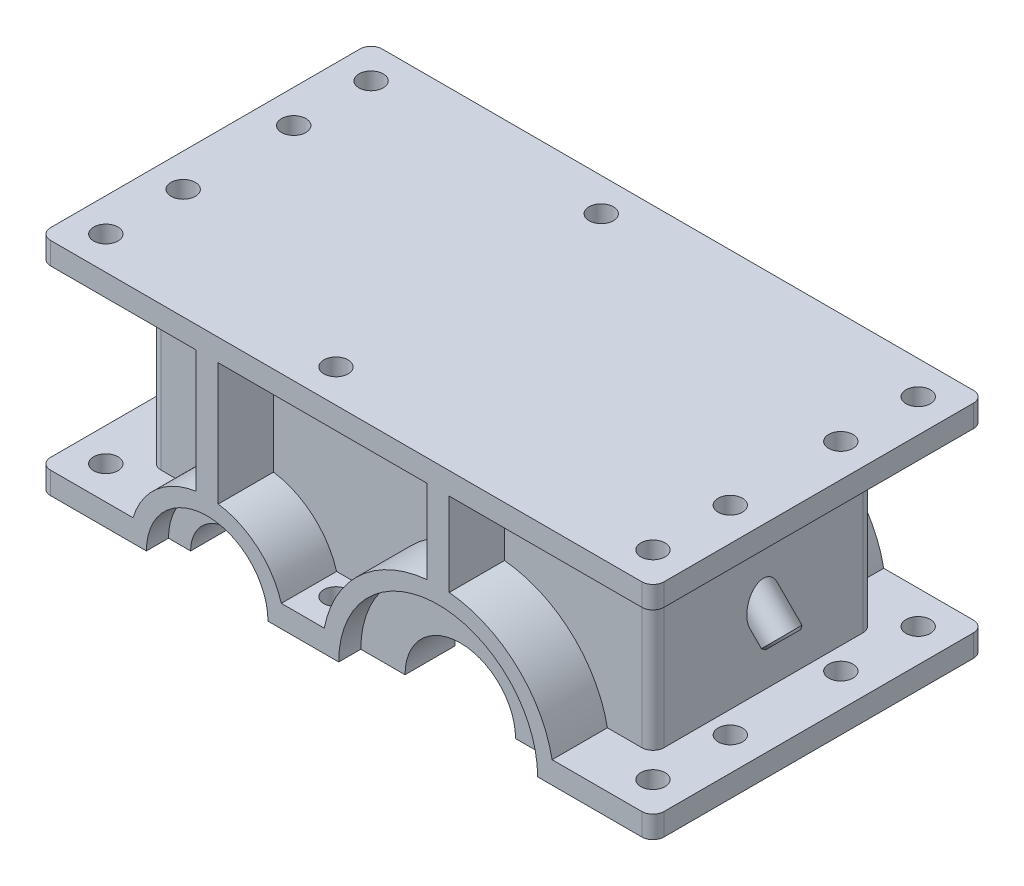
SolidWorks part; units mm, degrees
ref_plane "Front Plane" through (0, 0, 0) normal (0, 0, 1) x (1, 0, 0)
ref_plane "Top Plane" through (0, 0, 0) normal (0, 1, 0) x (1, 0, 0)
ref_plane "Right Plane" through (0, 0, 0) normal (1, 0, 0) x (0, 0, -1)
sketch "Sketch1" plane through (0, 0, 0) normal (0, 0, 1) x (1, 0, 0)
  line L0 (-200, 0) -> (255, 0) construction
  line L1 (0, 200) -> (0, -201.1908) construction
  line L2 (-200, 200) -> (-200, 0)
  line L3 (255, 0) -> (255, 200)
  line L4 (-14.196, 0) -> (-14.196, 143.4811) construction
  line L5 (-200, 0) -> (255, 0)
  line L6 (255, 200) -> (-200, 200)
  circle A0 centre (-98.2783, 0) radius 84 construction
  circle A1 centre (110.7228, 0) radius 125 construction
  dimension "D1" = 250
  dimension "D2" = 110.7228
  dimension "D3" = 168
  dimension "D4" = 209.0011
  dimension "D5" = 200
  dimension "D7" = 200
  dimension "D8" = 255
extrude "Boss-Extrude1" add sketch "Sketch1" along normal mid plane 200
shell "Shell1" thickness 15
sketch "Sketch2" plane through (0, 0, 0) normal (0, 1, 0) x (1, 0, 0)
  line L8 (-114.9858, 100) -> (-200, 100)
  line L9 (54.3355, 100) -> (-114.9858, 100)
  line L10 (255, 100) -> (54.3355, 100)
  line L11 (255, -100) -> (255, 100)
  line L12 (54.3355, -100) -> (255, -100)
  line L13 (-114.9858, -100) -> (54.3355, -100)
  line L14 (-200, -100) -> (-114.9858, -100)
  line L15 (-200, -100) -> (-200, 100)
  line L16 (-114.9858, 150) -> (-250, 150)
  line L17 (-250, -150) -> (-250, 150)
  line L18 (-250, -150) -> (-114.9858, -150)
  line L19 (-114.9858, -150) -> (54.3355, -150)
  line L20 (54.3355, -150) -> (305, -150)
  line L21 (305, -150) -> (305, 150)
  line L22 (305, 150) -> (54.3355, 150)
  line L23 (54.3355, 150) -> (-114.9858, 150)
  dimension "D1" = 50
extrude "Boss-Extrude2" add sketch "Sketch2" along normal blind 20
sketch "Sketch3" plane through (0, 0, 100) normal (0, 0, 1) x (1, 0, 0)
  line L0 (-168.2783, 0) -> (-28.2783, 0)
  line L1 (5.7228, 0) -> (215.7228, 0)
  arc A0 (-28.2783, 0) -> (-168.2783, 0) centre (-98.2783, 0) ccw
  arc A1 (215.7228, 0) -> (5.7228, 0) centre (110.7228, 0) ccw
  line M2 (-200, 20) -> (255, 20)
  dimension "D1" = 105
  dimension "D2" = 70
extrude "Boss-Extrude3" add sketch "Sketch3" along normal blind 50 contours A1 M2 | A0 M2
sketch "Sketch4" plane through (0, 0, 150) normal (0, 0, 1) x (1, 0, 0)
  line L0 (-98.2783, 55) -> (-98.2783, 70) construction
  line L1 (110.7228, 90) -> (110.7228, 105) construction
  circle A0 centre (110.7228, 0) radius 90
  circle A1 centre (-98.2783, 0) radius 55
  arc A2 (-31.1963, 20) -> (-165.3604, 20) centre (-98.2783, 0) ccw construction
  arc A3 (213.8004, 20) -> (7.6451, 20) centre (110.7228, 0) ccw construction
  dimension "D1" = 110
  dimension "D2" = 180
extrude "Cut-Extrude1" cut sketch "Sketch4" against normal blind 20
mirror "Mirror1" about plane through (0, 0, 0) normal (0, 0, 1) of "Cut-Extrude1", "Boss-Extrude3"
sketch "Sketch5" plane through (0, 0, 130) normal (0, 0, 1) x (1, 0, 0)
  circle A0 centre (-98.2783, 0) radius 35
  circle A1 centre (110.7228, 0) radius 50
  dimension "D1" = 70
  dimension "D2" = 100
extrude "Cut-Extrude3" cut sketch "Sketch5" against normal through all
fillet "Fillet1" radius 10 8 edges at (305, 10, 150) (305, 10, -150) (-250, 10, -150) (-250, 10, 150) (-200, 110, -100) (255, 110, -100) (255, 110, 100) (-200, 110, 100)
sketch "Sketch6" plane through (0, 20, 0) normal (0, 1, 0) x (1, 0, 0)
  line L0 (-250, 0) -> (305, 0) construction
  line L1 (-220, 120) -> (-220, 150) construction
  line L2 (-165.3604, 150) -> (-240, 150) construction
  line L3 (-220, 120) -> (-250, 120) construction
  line L4 (-250, 140) -> (-250, -140) construction
  line L5 (-220, -120) -> (-250, -120) construction
  line L6 (-220, -120) -> (-220, -150) construction
  line L7 (305, -140) -> (305, 140) construction
  line L8 (27.5, 0) -> (27.5, 385.3878) construction
  line L9 (275, -120) -> (275, -150) construction
  line L10 (275, -120) -> (305, -120) construction
  line L11 (275, 120) -> (305, 120) construction
  line L12 (275, 120) -> (275, 150) construction
  line L13 (-11.7756, 100) -> (-11.7756, 150) construction
  line L14 (7.6451, 100) -> (-31.1963, 100) construction
  line L15 (7.6451, 150) -> (-31.1963, 150) construction
  line L16 (-250, 120) -> (305, 120) construction
  circle A0 centre (-220, 120) radius 11
  circle A1 centre (-220, 50) radius 11
  circle A2 centre (-220, -50) radius 11
  circle A3 centre (-220, -120) radius 11
  circle A4 centre (275, -120) radius 11
  circle A5 centre (275, -50) radius 11
  circle A6 centre (275, 50) radius 11
  circle A7 centre (275, 120) radius 11
  circle A8 centre (-11.7756, 120) radius 11
  circle A9 centre (-11.7756, -120) radius 11
  dimension "D1" = 22
  dimension "D4" = 22
  dimension "D6" = 22
  dimension "D2" = 30
  dimension "D3" = 30
  dimension "D5" = 70
extrude "Cut-Extrude4" cut sketch "Sketch6" against normal blind 30
sketch "Sketch7" plane through (0, 200, 0) normal (0, 1, 0) x (1, 0, 0)
  line L0 (-165.3604, 150) -> (-240, 150) construction
  line L1 (-250, 140) -> (-250, -140) construction
  line L2 (-240, -150) -> (-165.3604, -150) construction
  line L3 (-165.3604, -150) -> (-31.1963, -150) construction
  line L4 (245, 100) -> (-190, 100)
  line L5 (-200, 90) -> (-200, -90)
  line L6 (-190, -100) -> (245, -100)
  line L7 (255, -90) -> (255, 90)
  line L8 (245, 100) -> (-190, 100)
  line L9 (-200, 90) -> (-200, -90)
  line L10 (-190, -100) -> (245, -100)
  line L11 (255, -90) -> (255, 90)
  line L12 (-31.1963, -150) -> (7.6451, -150) construction
  line L13 (7.6451, -150) -> (213.8004, -150) construction
  line L14 (213.8004, -150) -> (295, -150) construction
  line L15 (305, -140) -> (305, 140) construction
  line L16 (295, 150) -> (213.8004, 150) construction
  line L17 (213.8004, 150) -> (7.6451, 150) construction
  line L18 (7.6451, 150) -> (-31.1963, 150) construction
  line L19 (-31.1963, 150) -> (-165.3604, 150) construction
  line L20 (-165.3604, 150) -> (-240, 150)
  line L21 (-250, 140) -> (-250, -140)
  line L22 (-240, -150) -> (-165.3604, -150)
  line L23 (-165.3604, -150) -> (-31.1963, -150)
  line L24 (-31.1963, -150) -> (7.6451, -150)
  line L25 (7.6451, -150) -> (213.8004, -150)
  line L26 (213.8004, -150) -> (295, -150)
  line L27 (305, -140) -> (305, 140)
  line L28 (295, 150) -> (213.8004, 150)
  line L29 (213.8004, 150) -> (7.6451, 150)
  line L30 (7.6451, 150) -> (-31.1963, 150)
  line L31 (-31.1963, 150) -> (-165.3604, 150)
  arc A0 (-240, 150) -> (-250, 140) centre (-240, 140) ccw construction
  arc A1 (-250, -140) -> (-240, -150) centre (-240, -140) ccw construction
  arc A2 (295, -150) -> (305, -140) centre (295, -140) ccw construction
  arc A3 (305, 140) -> (295, 150) centre (295, 140) ccw construction
  arc A4 (-190, 100) -> (-200, 90) centre (-190, 90) ccw
  arc A5 (-200, -90) -> (-190, -100) centre (-190, -90) ccw
  arc A6 (245, -100) -> (255, -90) centre (245, -90) ccw
  arc A7 (255, 90) -> (245, 100) centre (245, 90) ccw
  arc A8 (-190, 100) -> (-200, 90) centre (-190, 90) ccw
  arc A9 (-200, -90) -> (-190, -100) centre (-190, -90) ccw
  arc A10 (245, -100) -> (255, -90) centre (245, -90) ccw
  arc A11 (255, 90) -> (245, 100) centre (245, 90) ccw
  arc A12 (-240, 150) -> (-250, 140) centre (-240, 140) ccw
  arc A13 (-250, -140) -> (-240, -150) centre (-240, -140) ccw
  arc A14 (295, -150) -> (305, -140) centre (295, -140) ccw
  arc A15 (305, 140) -> (295, 150) centre (295, 140) ccw
  circle A16 centre (-220, 120) radius 11 construction
  circle A17 centre (-220, 50) radius 11 construction
  circle A18 centre (-220, -50) radius 11 construction
  circle A19 centre (-220, -120) radius 11 construction
  circle A20 centre (-11.7756, -120) radius 11 construction
  circle A21 centre (-11.7756, 120) radius 11 construction
  circle A22 centre (275, 120) radius 11 construction
  circle A23 centre (275, 50) radius 11 construction
  circle A24 centre (275, -50) radius 11 construction
  circle A25 centre (275, -120) radius 11 construction
  circle A26 centre (-220, 120) radius 11
  circle A27 centre (-220, 50) radius 11
  circle A28 centre (-220, -50) radius 11
  circle A29 centre (-220, -120) radius 11
  circle A30 centre (-11.7756, -120) radius 11
  circle A31 centre (-11.7756, 120) radius 11
  circle A32 centre (275, 120) radius 11
  circle A33 centre (275, 50) radius 11
  circle A34 centre (275, -50) radius 11
  circle A35 centre (275, -120) radius 11
  dimension "D1" = 0
extrude "Boss-Extrude4" add sketch "Sketch7" against normal blind 20
ref_plane "Plane1" through (110.72, 0, 0) normal (1, 0, 0) x (0, 0, -1)
ref_plane "Plane2" through (-98.28, 0, 0) normal (1, 0, 0) x (0, 0, -1)
sketch "Sketch8" plane through (110.72, 0, 0) normal (1, 0, 0) x (0, 0, -1)
  line L0 (100, 100) -> (150, 100)
  line L1 (100, 180) -> (100, 20) construction
  line L2 (150, 20) -> (150, 105) construction
  line L3 (150, 100) -> (150, 184.7546)
  line L4 (150, 184.7546) -> (95.8916, 184.7546)
  line L5 (95.8916, 184.7546) -> (100, 100)
  line L6 (0, 275.8668) -> (0, -86.1959) construction
  line L7 (-95.8916, 184.7546) -> (-100, 100)
  line L8 (-150, 184.7546) -> (-95.8916, 184.7546)
  line L9 (-150, 100) -> (-150, 184.7546)
  line L10 (-100, 100) -> (-150, 100)
extrude "Boss-Extrude5" add sketch "Sketch8" along normal mid plane 20
sketch "Sketch9" plane through (-98.28, 0, 0) normal (1, 0, 0) x (0, 0, -1)
  line L0 (150, 180) -> (150, 200) construction
  line L3 (150, 185.669) -> (94.5689, 185.669)
  line L4 (150, 185.669) -> (150, 58.4902)
  line L6 (150, 58.4902) -> (94.5689, 58.4902)
  line L7 (0, -71.1468) -> (0, 262.5866) construction
  line L8 (94.5689, 185.669) -> (94.5689, 58.4902)
  line L9 (-94.5689, 185.669) -> (-94.5689, 58.4902)
  line L10 (-150, 58.4902) -> (-94.5689, 58.4902)
  line L11 (-150, 185.669) -> (-150, 58.4902)
  line L13 (-150, 185.669) -> (-94.5689, 185.669)
extrude "Boss-Extrude6" add sketch "Sketch9" along normal mid plane 20
sketch "Sketch10" plane through (0, 0, 0) normal (0, 0, 1) x (1, 0, 0)
  line L0 (161.5532, 180) -> (323.8586, 17.6946) construction
  line L1 (120.72, 180) -> (245, 180) construction
  line L2 (120.72, 180) -> (295, 180) construction
  line L4 (243.882, 118.8844) -> (283.5325, 79.234)
  line L5 (172.1598, 190.6066) -> (334.4652, 28.3012) construction
  line L7 (243.882, 118.8844) -> (233.1557, 108.3975)
  line L8 (283.5325, 79.234) -> (272.9259, 68.6274)
  line L9 (233.1557, 108.3975) -> (272.9259, 68.6274)
  dimension "D1" = 45
  dimension "D3" = 15
revolve "Revolve1" add sketch "Sketch10" angle 360 about L0
sketch "Sketch11" plane through (102.1493, -102.1493, 0) normal (0.7071, -0.7071, 0) x (0, 0, -1)
  line L0 (0, 241.5146) -> (0, 275.3384) construction
  circle A0 centre (0, 241.5146) radius 9
  dimension "D1" = 18
extrude "Cut-Extrude5" cut sketch "Sketch11" against normal blind 70
sketch "Sketch12" plane through (0, 0, 0) normal (0, -1, 0) x (1, 0, 0)
  line L0 (160.7228, 85) -> (160.7228, -85)
  line L12 (305, -140) -> (305, 140)
  line L13 (295, 150) -> (200.7228, 150)
  line L14 (200.7228, 150) -> (200.7228, 130)
  line L15 (200.7228, 130) -> (160.7228, 130)
  line L16 (160.7228, 130) -> (160.7228, 85)
  line L17 (160.7228, 85) -> (240, 85)
  line L18 (240, 85) -> (240, -85)
  line L19 (240, -85) -> (160.7228, -85)
  line L20 (160.7228, -85) -> (160.7228, -130)
  line L21 (160.7228, -130) -> (200.7228, -130)
  line L22 (200.7228, -130) -> (200.7228, -150)
  line L23 (200.7228, -150) -> (295, -150)
  line L29 (160.7228, 85) -> (240, 85)
  line L30 (240, 85) -> (240, -85)
  line L31 (240, -85) -> (160.7228, -85)
  arc A2 (305, 140) -> (295, 150) centre (295, 140) ccw
  arc A3 (295, -150) -> (305, -140) centre (295, -140) ccw
  dimension "D1" = 0
extrude "Cut-Extrude6" cut sketch "Sketch12" against normal blind 130
chamfer "Chamfer1" distance 2 angle 45 1 edges at (262.3193, 58.0208, 0)
